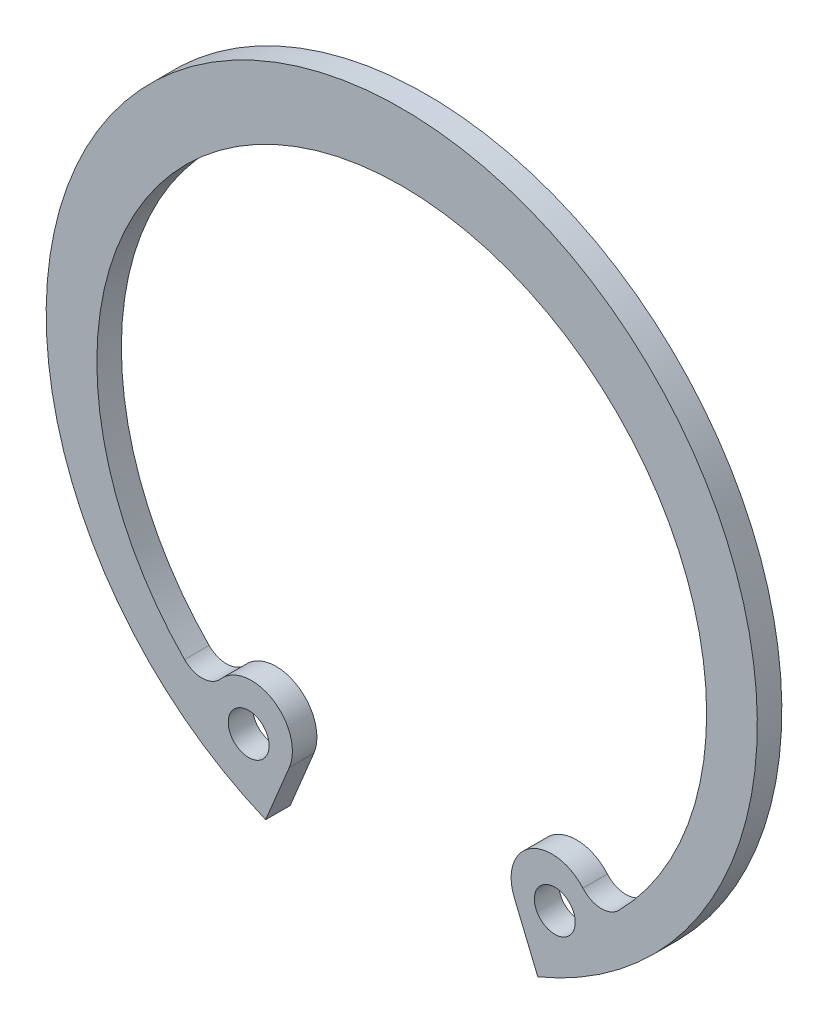
from build123d import *

# Parameters (mm, degrees)
EXTRUDE_962_DEPTH      = 0.75
EXTRUDE_962_DEPTH_BACK = 0.75
SKETCH_1_R             = 1.25


with BuildPart() as part:
    # 草图1 → Extrude 962 (new, two sides: drawn at the far end of the back side and taken through both)
    with BuildSketch(Plane.XY.offset(-EXTRUDE_962_DEPTH_BACK)):
        with BuildLine():
            Line((-6.879499755, -16.608581611), (-8.323364654, -20.094379832))
            ThreePointArc((-8.323364654, -20.094379832), (0, 21.75), (8.323364654, -20.094379832))
            Line((8.323364654, -20.094379832), (6.879499755, -16.608581611))
            ThreePointArc((6.879499755, -16.608581611), (7.876948304, -13.523963446), (11.081029231, -14.017560694))
            ThreePointArc((11.081029231, -14.017560694), (12.16700015, -14.536168573), (13.28459359, -14.08976979))
            ThreePointArc((13.28459359, -14.08976979), (0, 17.65), (-13.28459359, -14.08976979))
            ThreePointArc((-13.28459359, -14.08976979), (-12.16700015, -14.536168573), (-11.081029231, -14.017560694))
            ThreePointArc((-11.081029231, -14.017560694), (-7.876948304, -13.523963446), (-6.879499755, -16.608581611))
        make_face()
        with Locations((-9.363022706, -16.071521577)):
            Circle(SKETCH_1_R, mode=Mode.SUBTRACT)
        with Locations(Location((9.363022706, -16.071521577, 0), (0, 0, 180))):
            Circle(SKETCH_1_R, mode=Mode.SUBTRACT)
    extrude(amount=EXTRUDE_962_DEPTH + EXTRUDE_962_DEPTH_BACK)


solid = part.part
